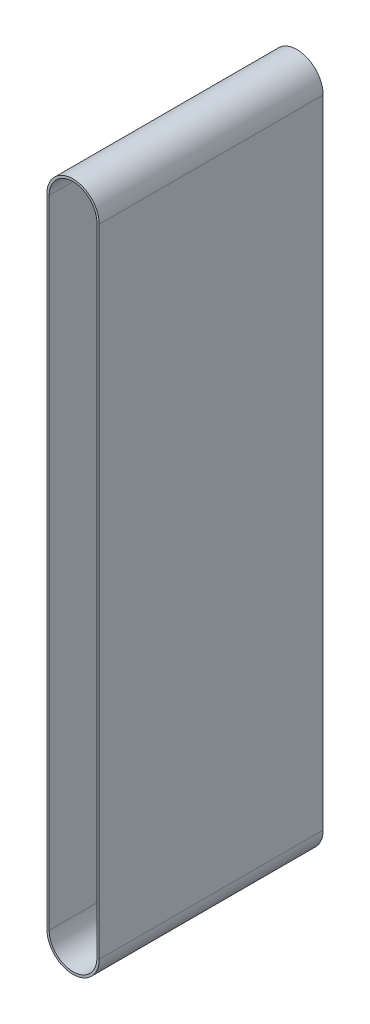
from build123d import *

# Parameters (mm, degrees)
EXTRUDE_1_DEPTH = 95


with BuildPart() as part:
    # 草图2 → 拉伸-薄壁1 (new, symmetric)
    with BuildSketch(Plane.XY):
        with BuildLine():
            Line((22.25, 540), (22.25, 0))
            ThreePointArc((22.25, 0), (0, -22.25), (-22.25, 0))
            Line((-22.25, 0), (-22.25, 540))
            ThreePointArc((-22.25, 540), (0, 562.25), (22.25, 540))
        make_face()
        with BuildLine():
            Line((20.25, 540), (20.25, 0))
            ThreePointArc((20.25, 0), (0, -20.25), (-20.25, 0))
            Line((-20.25, 0), (-20.25, 540))
            ThreePointArc((-20.25, 540), (0, 560.25), (20.25, 540))
        make_face(mode=Mode.SUBTRACT)
    extrude(amount=EXTRUDE_1_DEPTH, both=True)


solid = part.part
